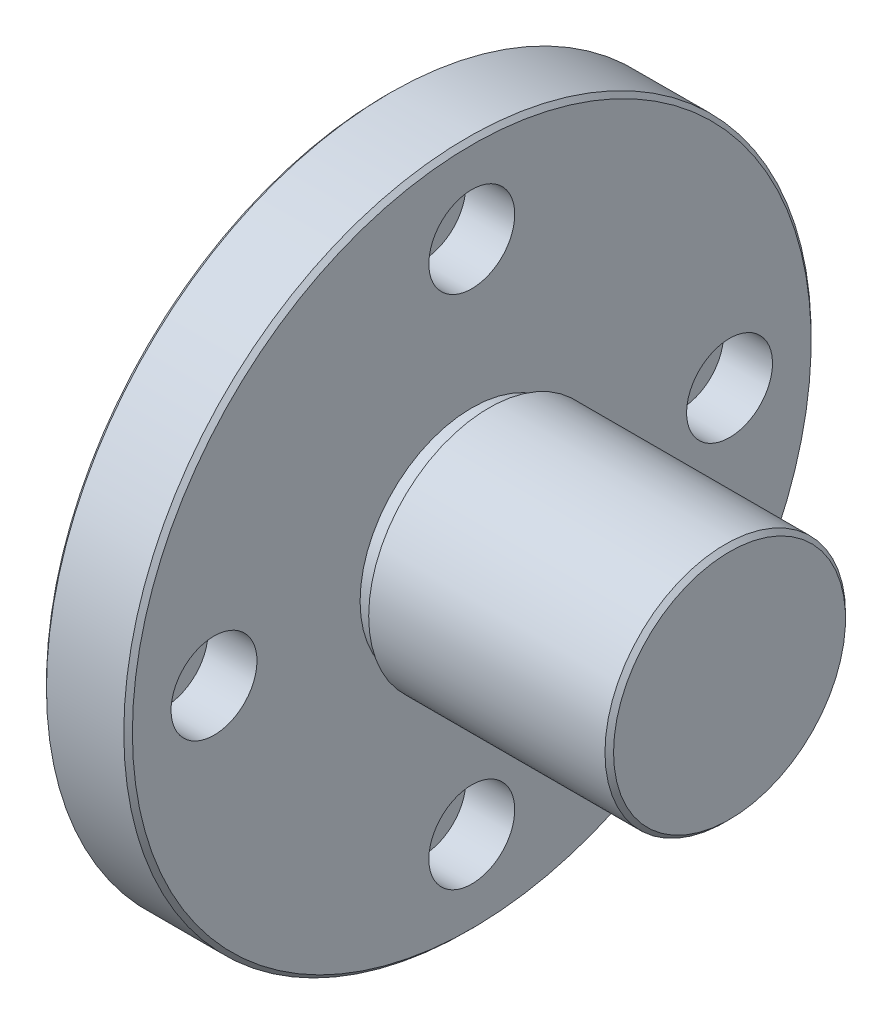
SolidWorks part; units mm, degrees
material "6061"
ref_plane "前视基准面" through (0, 0, 0) normal (0, 0, 1) x (1, 0, 0)
ref_plane "上视基准面" through (0, 0, 0) normal (0, 1, 0) x (1, 0, 0)
ref_plane "右视基准面" through (0, 0, 0) normal (1, 0, 0) x (0, 0, -1)
sketch "草图2" plane through (0, 0, 0) normal (0, 0, 1) x (1, 0, 0)
  line L0 (0, 0) -> (40, 0) construction
  line L1 (0, 0) -> (0, 40)
  line L2 (0, 40) -> (10, 40)
  line L3 (10, 40) -> (10, 13)
  line L4 (10, 13) -> (12, 13)
  line L5 (12, 13) -> (12, 14)
  line L6 (12, 14) -> (40, 14)
  line L7 (40, 14) -> (40, 0)
  line L8 (0, 0) -> (40, 0)
  dimension "D1" = 80
  dimension "D2" = 28
  dimension "D3" = 10
  dimension "D4" = 2
  dimension "D5" = 40
  dimension "D6" = 26
revolve "旋转1" add sketch "草图2" angle 360 about L0
cosmetic thread "装饰螺纹线1" parameters "D2"=26.9
cosmetic thread "装饰螺纹线2" parameters "D1"=5, "D2"=6.647
hole_wizard "Ø9.0 (9) 直径孔1" positions "草图4" profile "草图3" hole size "Ø9.0" standard "GB"
sketch "草图4" plane through (0, 0, 0) normal (-1, 0, 0) x (0, 0, 1)
  point P0 (0, 0)
sketch "草图3" plane through (0, 0, 0) normal (0, 1, 0) x (0, 0, 1)
  line L0 (0, 0) -> (0, 40)
  line L1 (0, 40) -> (4.5, 40)
  line L2 (4.5, 40) -> (4.5, 0)
  line L5 (4.5, 0) -> (0, 0)
  line L11 (0, -6.35) -> (0, 107.95) construction
  dimension "通孔孔直径" = 9
  dimension "通孔孔深度" = 40
sketch "草图5" [suppressed] plane through (40, 0, 0) normal (1, 0, 0) x (0, 0, -1)
  circle A0 centre (0, 0) radius 8
  dimension "D1" = 16
extrude "切除-拉伸1" [suppressed] cut sketch "草图5" against normal blind 6
chamfer "倒角1" distance 0.5 angle 45 3 edges at (10, 0, 40) (0, 0, 40) (40, 0, 14)
hole_wizard "打孔尺寸(%根据)内六角圆柱头螺钉的类型1" positions "草图6" profile "草图7" counterbore size "M5" standard "GB"
sketch "草图6" plane through (10, 0, 0) normal (1, 0, 0) x (0, 0, -1)
  circle A0 centre (0, 0) radius 30
  point P0 (0, 30)
  dimension "D1" = 60
sketch "草图7" plane through (10, 30, 0) normal (0, 1, 0) x (0, 0, -1)
  line L0 (0, 0) -> (0, 13.1524)
  line L1 (0, 13.1524) -> (2.75, 11.5)
  line L2 (2.75, 11.5) -> (2.75, 5.7)
  line L3 (2.75, 5.7) -> (5, 5.7)
  line L4 (5, 5.7) -> (5, 0)
  line L5 (5, 0) -> (0, 0)
  line L10 (0, 13.1524) -> (-2.75, 11.5) construction
  line L11 (0, -6.35) -> (0, 107.95) construction
  dimension "孔直径" = 5.5
  dimension "孔深度" = 11.5
  dimension "柱形沉头孔直径" = 10
  dimension "柱形沉头孔深度" = 5.7
  dimension "导头角度" = 118
pattern_circular "阵列(圆周)1" count 4 over 360 about axis through (0, 0, 0) along (1, 0, 0) of "打孔尺寸(%根据)内六角圆柱头螺钉的类型1"
